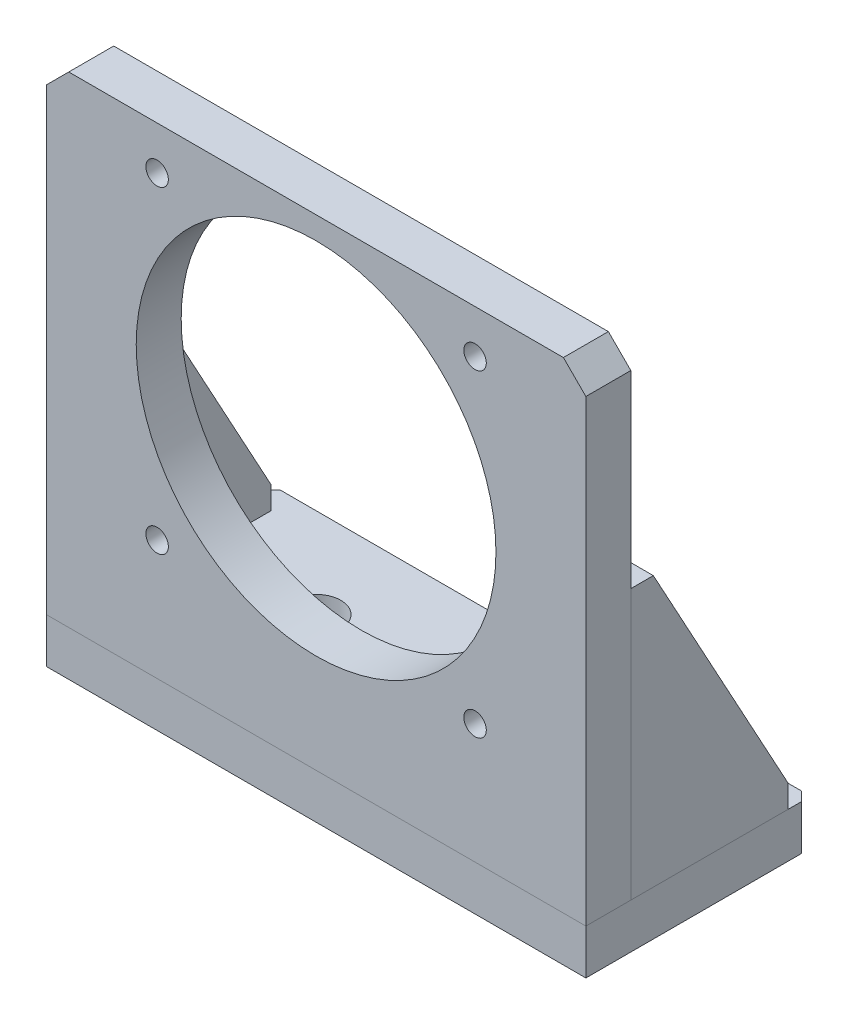
SolidWorks part; units mm, degrees
material "45#"
ref_plane "前基準面" through (0, 0, 0) normal (0, 0, 1) x (1, 0, 0)
ref_plane "上基準面" through (0, 0, 0) normal (0, 1, 0) x (1, 0, 0)
ref_plane "右基準面" through (0, 0, 0) normal (1, 0, 0) x (0, 0, -1)
sketch "草图1" plane through (0, 0, 0) normal (0, 1, 0) x (1, 0, 0)
  line L1 (-60, -25) -> (60, -25)
  line L2 (-60, -25) -> (-60, 25)
  line L3 (-60, 25) -> (60, 25)
  line L4 (60, -25) -> (60, 25)
  line L5 (-60, -25) -> (60, 25) construction
  line L6 (-60, 25) -> (60, -25) construction
  point P0 (0, 0)
  dimension "D1" = 120
  dimension "D2" = 50
extrude "凸台-拉伸1" add sketch "草图1" along normal mid plane 10
sketch "草图2" plane through (0, 5, 0) normal (0, 1, 0) x (1, 0, 0)
  line L0 (-60, 25) -> (-60, -25) construction
  line L1 (60, -25) -> (-60, -25)
  line L2 (60, -25) -> (60, -15)
  line L3 (60, -15) -> (-60, -15)
  line L4 (-60, -25) -> (-60, -15)
  dimension "D1" = 10
extrude "凸台-拉伸2" add sketch "草图2" along normal blind 107 separate body
chamfer "倒角1" distance 5 angle 45 2 edges at (60, 112, 20) (-60, 112, 20)
chamfer "倒角2" distance 2 angle 45 2 edges at (-60, 0, -25) (60, 0, -25)
sketch "草图3" plane through (-60, 0, 0) normal (-1, 0, 0) x (0, 0, 1)
  line L0 (15, 65) -> (10, 65)
  line L1 (15, 107) -> (15, 5) construction
  line L2 (10, 65) -> (-20, 10)
  line L3 (-20, 10) -> (-20, 5)
  line L4 (-23, 5) -> (25, 5) construction
  line L5 (-20, 5) -> (15, 5)
  line L6 (15, 5) -> (15, 65)
  line L7 (-25, -5) -> (-25, 5) construction
  dimension "D1" = 5
  dimension "D2" = 60
  dimension "D3" = 5
extrude "凸台-拉伸3" add sketch "草图3" against normal blind 5 separate body
mirror "镜向1" about plane through (0, 0, 0) normal (1, 0, 0) of bodies 103
sketch "草图4" plane through (0, 0, 25) normal (0, 0, 1) x (1, 0, 0)
  line L0 (-60, -5) -> (60, -5) construction
  circle A0 centre (0, 67) radius 40
  dimension "D1" = 80
  dimension "D2" = 72
extrude "切除-拉伸1" cut sketch "草图4" against normal up to surface (10 mm away) up to face at (0, 74.6667, 15)
hole_wizard "M10 间隙孔1" positions "草图5" profile "草图6" hole size "M10" standard "GB" end condition through all
sketch "草图5" plane through (0, 5, 0) normal (0, 1, 0) x (1, 0, 0)
  line L0 (0, 0) -> (0, 30.7245) construction
  line L2 (58, 25) -> (-58, 25) construction
  point P0 (30, 5)
  point P8 (-30, 5)
  dimension "D1" = 60
  dimension "D2" = 20
sketch "草图6" plane through (30, 5, -5) normal (1, 0, 0) x (0, 0, 1)
  line L0 (0, 0) -> (0, 10)
  line L1 (0, 10) -> (5.5, 10)
  line L2 (5.5, 10) -> (5.5, 0)
  line L5 (5.5, 0) -> (0, 0)
  line L11 (0, -6.35) -> (0, 107.95) construction
  dimension "通孔孔直径" = 11
  dimension "通孔孔深度" = 10
hole_wizard "M6 螺纹孔1" positions "草图7" profile "草图8" tap size "M6" standard "GB"
sketch "草图7" plane through (0, 0, 25) normal (0, 0, 1) x (1, 0, 0)
  circle A0 centre (0, 67) radius 50 construction
  point P0 (-35.3553, 102.3553)
  point P6 (35.3553, 102.3553)
  point P7 (35.3553, 31.6447)
  point P8 (-35.3553, 31.6447)
  dimension "D2" = 100
  dimension "D1" = 4
sketch "草图8" plane through (-35.3553, 102.3553, 25) normal (1, 0, 0) x (0, -1, 0)
  line L0 (0, 0) -> (0, 16.5022)
  line L1 (0, 16.5022) -> (2.5, 15)
  line L2 (2.5, 15) -> (2.5, 0)
  line L5 (2.5, 0) -> (0, 0)
  line L10 (0, 16.5022) -> (-2.5, 15) construction
  line L11 (0, -6.35) -> (0, 107.95) construction
  dimension "螺纹孔钻头直径" = 5
  dimension "螺纹孔钻头深度" = 15
  dimension "导头角度" = 118
cosmetic thread "孔螺蚊线1" parameters "D1"=10, "D2"=6
cosmetic thread "孔螺蚊线2" parameters "D1"=10, "D2"=6
cosmetic thread "孔螺蚊线3" parameters "D1"=10, "D2"=6
cosmetic thread "孔螺蚊线4" parameters "D1"=10, "D2"=6
